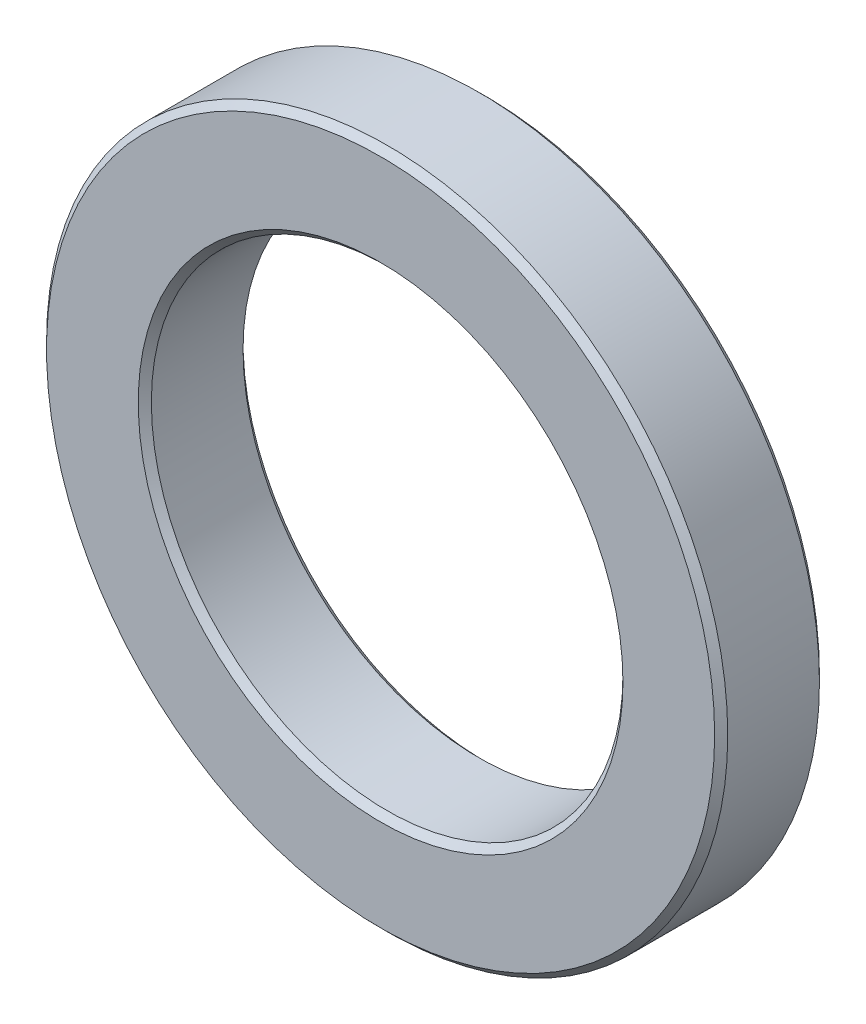
SolidWorks part; units mm, degrees
ref_plane "Front Plane" through (0, 0, 0) normal (0, 0, 1) x (1, 0, 0)
ref_plane "Top Plane" through (0, 0, 0) normal (0, 1, 0) x (1, 0, 0)
ref_plane "Right Plane" through (0, 0, 0) normal (1, 0, 0) x (0, 0, -1)
sketch "Sketch1" plane through (0, 0, 0) normal (0, 0, 1) x (1, 0, 0)
  circle A0 centre (0, 0) radius 26
  circle A1 centre (0, 0) radius 18
extrude "Boss-Extrude1" add sketch "Sketch1" along normal blind 8
chamfer "Chamfer1" distance 0.5 angle 45 4 edges at (26, 0, 8) (26, 0, 0) (18, 0, 0) (18, 0, 8)
